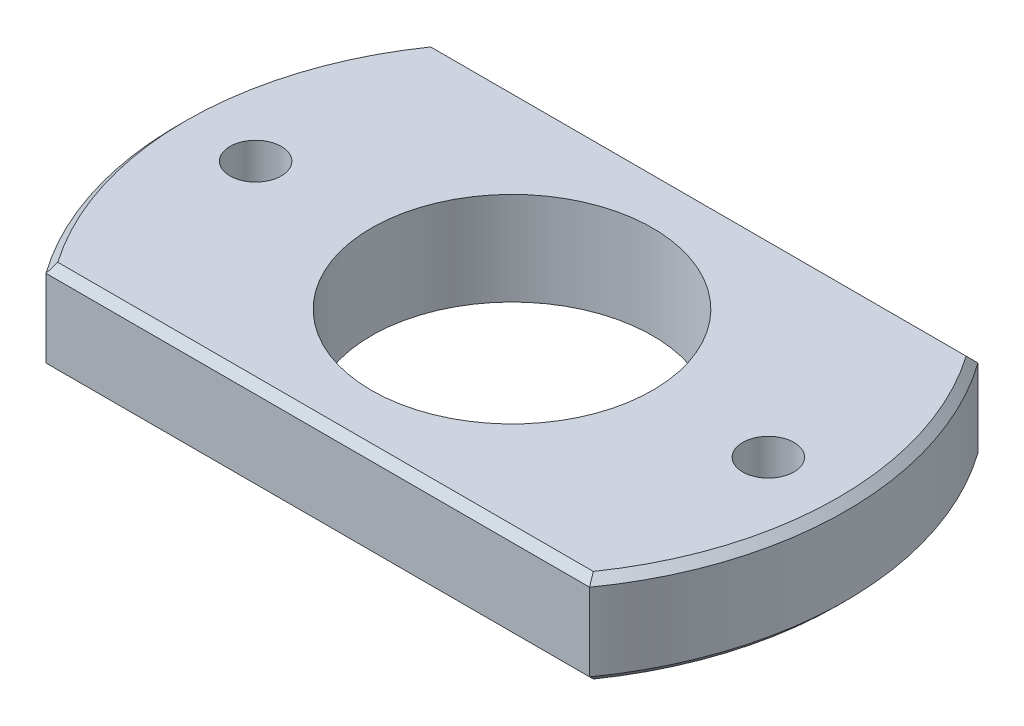
from build123d import *

# Parameters (mm, degrees)
SKETCH_1_R          = 21.5
EXTRUDE_1_DEPTH     = 6
HOLE_WIZARD_M4_1_D  = 3.3
SKETCH_5_W          = 80.188195039
SKETCH_5_H          = 23.165478567
SKETCH_5_W_2        = 146.4427716
SKETCH_5_H_2        = 26.907594335
CUT_EXTRUDE_1_DEPTH = 31.991934435
HOLE_WIZARD_M20_2_D = 18.1
CHAMFER_1_SIZE      = 0.5


with BuildPart() as part:
    # 草图1 → 凸台-拉伸1 (new body)
    with BuildSketch(Plane(origin=(0, 0, 0), x_dir=(1, 0, 0), z_dir=(0, 1, 0))):
        with Locations(Location((0, 0, 0), (0, 0, 270))):
            Circle(SKETCH_1_R)
    extrude(amount=EXTRUDE_1_DEPTH)

    # M4 螺纹孔1 (through all)
    with Locations(Plane(origin=(0, 6, 0), x_dir=(1, 0, 0), z_dir=(0, 1, 0))):
        with Locations((-16.5, 0), (16.5, 0)):
            Hole(HOLE_WIZARD_M4_1_D / 2)

    # 草图5 → 切除-拉伸1 (cut, through all)
    with BuildSketch(Plane(origin=(0, 6, 0), x_dir=(1, 0, 0), z_dir=(0, 1, 0))):
        with Locations((-5.212232678, 24.082739284)):
            Rectangle(SKETCH_5_W, SKETCH_5_H)
        with Locations((21.5, -25.953797168)):
            Rectangle(SKETCH_5_W_2, SKETCH_5_H_2)
    extrude(amount=-CUT_EXTRUDE_1_DEPTH, mode=Mode.SUBTRACT)

    # M20 螺纹孔2 (through all)
    with Locations(Plane(origin=(0, 6, 0), x_dir=(1, 0, 0), z_dir=(0, 1, 0))):
        with Locations((0, 0)):
            Hole(HOLE_WIZARD_M20_2_D / 2)

    # 倒角1
    chamfer_1_edges = [part.edges().sort_by_distance(p)[0] for p in [
        (-21.5, 0, 0),
        (0, 0, -12.5),
        (-21.5, 6, 0),
        (0, 6, -12.5),
        (21.5, 0, 0),
        (0, 0, 12.5),
        (21.5, 6, 0),
        (0, 6, 12.5),
    ]]
    chamfer(chamfer_1_edges, length=CHAMFER_1_SIZE)


solid = part.part
